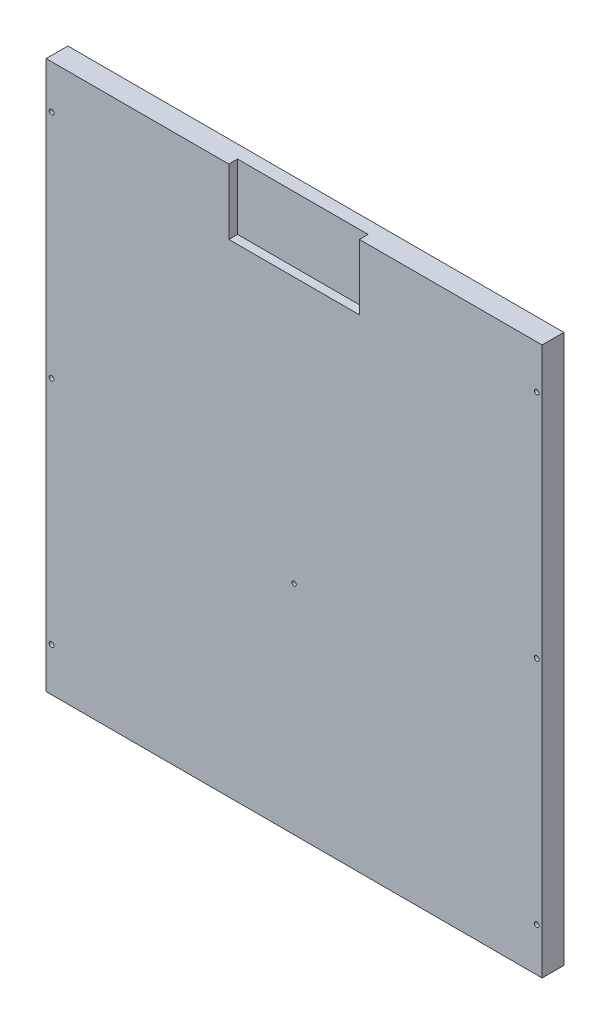
from build123d import *

# Parameters (mm, degrees)
SKETCH_1_W            = 1140
SKETCH_1_H            = 1260
EXTRUDE_1_DEPTH       = 50
SKETCH_2_R            = 5
SKETCH_2_R_2          = 5.5
SKETCH_2_W            = 300
SKETCH_2_H            = 300
CUT_EXTRUDE_986_DEPTH = 20


with BuildPart() as part:
    # 草图1 → 凸台-拉伸1 (new body)
    with BuildSketch(Plane.XY):
        Rectangle(SKETCH_1_W, SKETCH_1_H)
    extrude(amount=EXTRUDE_1_DEPTH)

    # 草图2 → Cut-Extrude 986 (cut)
    with BuildSketch(Plane.XY.offset(50)):
        with Locations((0, -130)):
            Circle(SKETCH_2_R)
        with Locations((557.5, -530)):
            Circle(SKETCH_2_R_2)
        with Locations((557.5, 0)):
            Circle(SKETCH_2_R_2)
        with Locations((557.5, 530)):
            Circle(SKETCH_2_R_2)
        with Locations(Location((-557.5, 530, 0), (0, 0, 180))):
            Circle(SKETCH_2_R_2)
        with Locations(Location((-557.5, 0, 0), (0, 0, 180))):
            Circle(SKETCH_2_R_2)
        with Locations(Location((-557.5, -530, 0), (0, 0, 180))):
            Circle(SKETCH_2_R_2)
        with Locations((0, 630)):
            Rectangle(SKETCH_2_W, SKETCH_2_H)
    extrude(amount=-CUT_EXTRUDE_986_DEPTH, mode=Mode.SUBTRACT)


solid = part.part
